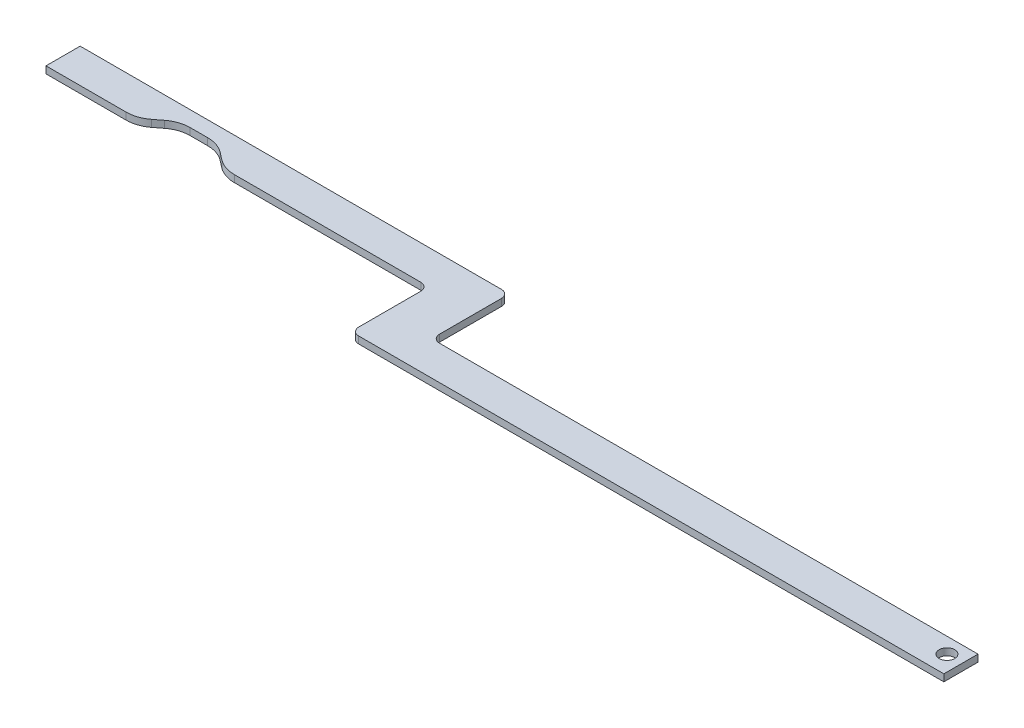
from build123d import *

# Parameters (mm, degrees)
SKETCH1_R           = 5
BOSS_EXTRUDE1_DEPTH = 4.5


with BuildPart() as part:
    # Sketch1 → Boss-Extrude1 (new body)
    with BuildSketch(Plane(origin=(0, 0, 0), x_dir=(1, 0, 0), z_dir=(0, 1, 0))):
        with BuildLine():
            Line((0, 0), (271.5, 0))
            ThreePointArc((271.5, 0), (275.035533906, -1.464466094), (276.5, -5))
            Line((276.5, -5), (276.5, -45))
            ThreePointArc((276.5, -45), (277.964466094, -48.535533906), (281.5, -50))
            Line((281.5, -50), (628.5, -50))
            Line((628.5, -50), (628.5, -72))
            Line((628.5, -72), (251.5, -72))
            ThreePointArc((251.5, -72), (247.964466094, -70.535533906), (246.5, -67))
            Line((246.5, -67), (246.5, -27))
            ThreePointArc((246.5, -27), (245.035533906, -23.464466094), (241.5, -22))
            Line((241.5, -22), (121.33715964, -22))
            ThreePointArc((121.33715964, -22), (114.86759563, -20.924712455), (109.09369578, -17.814474152))
            Line((109.09369578, -17.814474152), (104.40630422, -14.185525848))
            ThreePointArc((104.40630422, -14.185525848), (98.63240437, -11.075287545), (92.16284036, -10))
            Line((92.16284036, -10), (80.83715964, -10))
            ThreePointArc((80.83715964, -10), (74.36759563, -11.075287545), (68.59369578, -14.185525848))
            Line((68.59369578, -14.185525848), (63.90630422, -17.814474152))
            ThreePointArc((63.90630422, -17.814474152), (58.13240437, -20.924712455), (51.66284036, -22))
            Line((51.66284036, -22), (0, -22))
            Line((0, -22), (0, 0))
        make_face()
        with Locations(Location((618.5, -60, 0), (0, 0, 270))):
            Circle(SKETCH1_R, mode=Mode.SUBTRACT)
    extrude(amount=BOSS_EXTRUDE1_DEPTH)


solid = part.part
